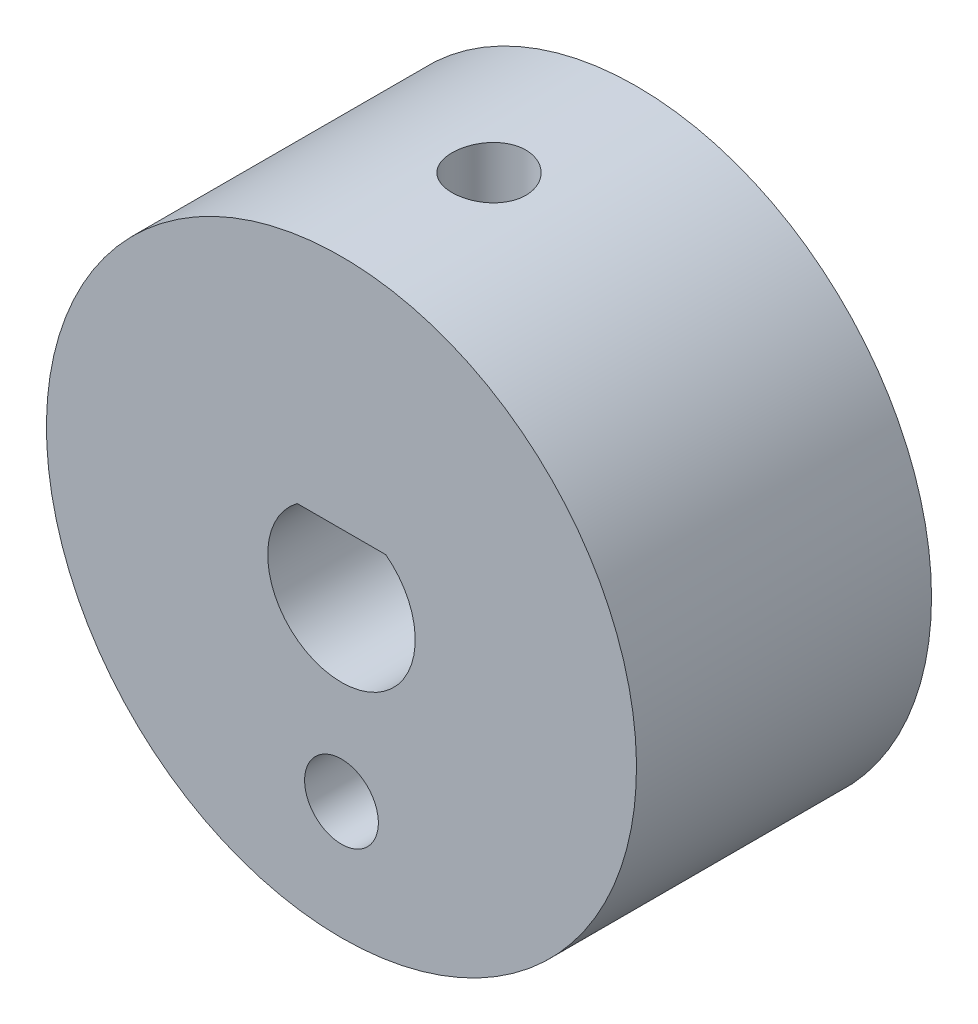
SolidWorks part; units mm, degrees
ref_plane "前视基准面" through (0, 0, 0) normal (0, 0, 1) x (1, 0, 0)
ref_plane "上视基准面" through (0, 0, 0) normal (0, 1, 0) x (1, 0, 0)
ref_plane "右视基准面" through (0, 0, 0) normal (1, 0, 0) x (0, 0, -1)
sketch "草图1" plane through (0, 0, 0) normal (0, 0, 1) x (1, 0, 0)
  line L0 (-1.5, 2) -> (1.5, 2) construction
  line L1 (-1.5, 2) -> (1.5, 2)
  arc A0 (-1.5, 2) -> (1.5, 2) centre (0, 0) ccw construction
  arc A1 (-1.5, 2) -> (1.5, 2) centre (0, 0) ccw
  circle A2 centre (0, 0) radius 10
  dimension "D1" = 20
extrude "凸台-拉伸1" add sketch "草图1" along normal up to surface (10 mm away)
sketch "草图2" plane through (0, 0, 10) normal (0, 0, 1) x (1, 0, 0)
  circle A1 centre (0, -6) radius 0.5
  dimension "D1" = 1
extrude "切除-拉伸1" cut sketch "草图2" against normal through all
ref_plane "基准面1" through (234.4117, 10, 915.57) normal (0, 1, 0) x (-1, 0, 0)
hole_wizard "M3 螺纹孔1" positions "草图10" profile "草图11" tap size "M3" standard "GB"
sketch "草图10" plane through (234.4117, 10, 915.57) normal (0, 1, 0) x (-1, 0, 0)
  line L1 (244.4117, -905.57) -> (224.4117, -905.57) construction
  point P0 (234.4117, -910.57)
  dimension "D1" = 5
sketch "草图11" plane through (0, 10, 5) normal (1, 0, 0) x (0, 0, 1)
  line L0 (0, 0) -> (0, 8)
  line L1 (0, 8) -> (1.25, 8)
  line L2 (1.25, 8) -> (1.25, 0)
  line L5 (1.25, 0) -> (0, 0)
  line L11 (0, -6.35) -> (0, 107.95) construction
  dimension "通孔螺纹孔钻头直径" = 2.5
  dimension "通孔螺纹孔钻头深度" = 8
cosmetic thread "孔螺蚊线1" parameters "D2"=3
hole_wizard "M3 螺纹孔2" positions "草图12" profile "草图13" tap size "M3" standard "GB" end condition through all
sketch "草图12" plane through (0, 0, 0) normal (0, 0, -1) x (-1, 0, 0)
  point P0 (0, -6)
sketch "草图13" plane through (0, -6, 0) normal (1, 0, 0) x (0, 1, 0)
  line L0 (0, 0) -> (0, 10)
  line L1 (0, 10) -> (1.25, 10)
  line L2 (1.25, 10) -> (1.25, 0)
  line L5 (1.25, 0) -> (0, 0)
  line L11 (0, -6.35) -> (0, 107.95) construction
  dimension "通孔螺纹孔钻头直径" = 2.5
  dimension "通孔螺纹孔钻头深度" = 10
cosmetic thread "孔螺蚊线2" parameters "D2"=3
